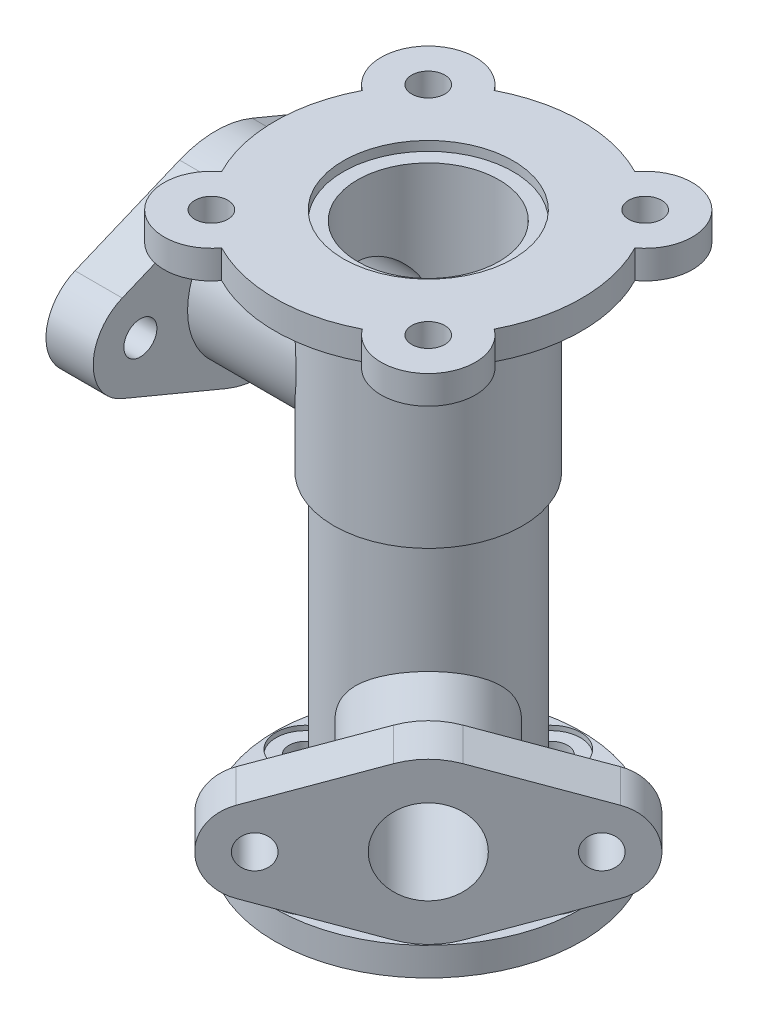
SolidWorks part; units mm, degrees
ref_plane "Front Plane" through (0, 0, 0) normal (0, 0, 1) x (1, 0, 0)
ref_plane "Top Plane" through (0, 0, 0) normal (0, 1, 0) x (1, 0, 0)
ref_plane "Right Plane" through (0, 0, 0) normal (1, 0, 0) x (0, 0, -1)
other "Configuration Table"
sketch "Sketch1" plane through (0, 0, 0) normal (0, 1, 0) x (1, 0, 0)
  circle A0 centre (0, 0) radius 32.5
  dimension "D1" = 65
extrude "Boss-Extrude1" add sketch "Sketch1" along normal blind 6
sketch "Sketch2" plane through (0, 6, 0) normal (0, 1, 0) x (1, 0, 0)
  circle A0 centre (0, 0) radius 18
  dimension "D1" = 36
extrude "Boss-Extrude2" add sketch "Sketch2" along normal blind 64
sketch "Sketch3" plane through (0, 70, 0) normal (0, 1, 0) x (1, 0, 0)
  circle A0 centre (0, 0) radius 20
  dimension "D1" = 40
extrude "Boss-Extrude3" add sketch "Sketch3" along normal blind 48
sketch "Sketch4" plane through (0, 118, 0) normal (0, 1, 0) x (1, 0, 0)
  line L0 (0, 44.6878) -> (0, 0) construction
  line L1 (0, 0) -> (32.5301, 32.5301) construction
  circle A0 centre (0, 0) radius 32.5
  circle A1 centre (22.981, 22.981) radius 10
  circle A5 centre (22.981, -22.981) radius 10
  circle A6 centre (-22.981, -22.981) radius 10
  circle A7 centre (-22.981, 22.981) radius 10
  point P16 (9.7122, 2.1531)
  point P17 (0, 0)
  circle M6 centre (0, 0) radius 20
  dimension "D1" = 65
  dimension "D2" = 20
  dimension "D3" = 45
  dimension "D4" = 4
extrude "Boss-Extrude4" add sketch "Sketch4" against normal blind 6 contours A0 A1 | A0 A1 | A7 A0 A6 A5 A1 M6 | M6 | A0 A5 | A0 A5 | A0 A6 | A0 A6
sketch "Sketch5" plane through (0, 0, 0) normal (1, 0, 0) x (0, 0, -1)
  line L0 (0, 90) -> (0, 0) construction
  circle A0 centre (0, 90) radius 16
  dimension "D2" = 32
  dimension "D1" = 90
extrude "Boss-Extrude5" add sketch "Sketch5" against normal blind 45
sketch "Sketch6" plane through (-45, 0, 0) normal (-1, 0, 0) x (0, 0, 1)
  line L0 (0, 139.4869) -> (0, 110) construction
  line L1 (0, 90) -> (47.008, 90) construction
  line L2 (7.6923, 71.5385) -> (29.8462, 80.7692)
  line L3 (7.6923, 108.4615) -> (29.8462, 99.2308)
  line L4 (-7.6923, 108.4615) -> (-29.8462, 99.2308)
  line L5 (-7.6923, 71.5385) -> (-29.8462, 80.7692)
  arc A0 (-7.6923, 71.5385) -> (7.6923, 71.5385) centre (0, 90) ccw
  arc A1 (29.8462, 80.7692) -> (29.8462, 99.2308) centre (26, 90) ccw
  arc A2 (-29.8462, 80.7692) -> (-29.8462, 99.2308) centre (-26, 90) cw
  arc A3 (7.6923, 108.4615) -> (-7.6923, 108.4615) centre (0, 90) ccw
  dimension "D1" = 40
  dimension "D2" = 20
  dimension "D3" = 52
extrude "Boss-Extrude6" add sketch "Sketch6" against normal blind 10
ref_plane "Plane1" through (0, 0, 0) normal (-0.7071, 0, 0.7071) x (0, -1, 0)
ref_plane "Plane2" through (0, 0, 0) normal (-0.7071, 0, -0.7071) x (0, -1, 0)
sketch "Sketch8" plane through (0, 0, 0) normal (-0.7071, 0, -0.7071) x (0, -1, 0)
  line L0 (-70, 0) -> (-6, 0) construction
  line L1 (-32, 0) -> (0, 0) construction
  circle A0 centre (-32, 0) radius 14
  dimension "D1" = 28
  dimension "D2" = 32
extrude "Boss-Extrude7" add sketch "Sketch8" against normal blind 45
sketch "Sketch9" plane through (31.8198, 0, 31.8198) normal (0.7071, 0, 0.7071) x (0.7071, 0, -0.7071)
  line L0 (0, 56.8043) -> (0, 32) construction
  line L1 (0, 32) -> (45.5222, 32) construction
  line L2 (5.2308, 15.8247) -> (28.7692, 23.4366)
  line L3 (5.2308, 48.1753) -> (28.7692, 40.5634)
  line L4 (-5.2308, 48.1753) -> (-28.7692, 40.5634)
  line L5 (-5.2308, 15.8247) -> (-28.7692, 23.4366)
  arc A0 (-5.2308, 15.8247) -> (5.2308, 15.8247) centre (0, 32) ccw
  arc A1 (28.7692, 23.4366) -> (28.7692, 40.5634) centre (26, 32) ccw
  arc A2 (-28.7692, 23.4366) -> (-28.7692, 40.5634) centre (-26, 32) cw
  arc A3 (5.2308, 48.1753) -> (-5.2308, 48.1753) centre (0, 32) ccw
  dimension "D1" = 18
  dimension "D2" = 34
  dimension "D3" = 52
extrude "Boss-Extrude8" add sketch "Sketch9" against normal blind 10
sketch "Sketch10" plane through (0, 0, 0) normal (0, -1, 0) x (1, 0, 0)
  circle A0 centre (0, 0) radius 13
  dimension "D1" = 26
extrude "Cut-Extrude1" cut sketch "Sketch10" against normal blind 70
sketch "Sketch11" plane through (31.8198, 0, 31.8198) normal (0.7071, 0, 0.7071) x (0.7071, 0, -0.7071)
  circle A0 centre (0, 32) radius 9
  dimension "D1" = 18
extrude "Cut-Extrude2" cut sketch "Sketch11" against normal blind 45
sketch "Sketch12" plane through (-45, 0, 0) normal (-1, 0, 0) x (0, 0, 1)
  circle A0 centre (0, 90) radius 11
  dimension "D1" = 22
extrude "Cut-Extrude3" cut sketch "Sketch12" against normal blind 45
sketch "Sketch13" plane through (0, 118, 0) normal (0, 1, 0) x (1, 0, 0)
  circle A0 centre (0, 0) radius 18
  dimension "D1" = 36
extrude "Cut-Extrude4" cut sketch "Sketch13" against normal blind 2
sketch "Sketch14" plane through (0, 116, 0) normal (0, 1, 0) x (1, 0, 0)
  circle A0 centre (0, 0) radius 15
  dimension "D1" = 30
extrude "Cut-Extrude5" cut sketch "Sketch14" against normal blind 36
sketch "Sketch15" plane through (0, 80, 0) normal (0, 1, 0) x (1, 0, 0)
  line L0 (0, -4.5826) -> (0, 4.5826) construction
  circle A0 centre (0, 0) radius 14
  dimension "D1" = 28
extrude "Cut-Extrude6" cut sketch "Sketch15" against normal blind 3
sketch "Sketch16" plane through (0, 118, 0) normal (0, 1, 0) x (1, 0, 0)
  circle A0 centre (22.981, 22.981) radius 3.5
  circle A1 centre (22.981, -22.981) radius 3.5
  circle A2 centre (-22.981, -22.981) radius 3.5
  circle A3 centre (-22.981, 22.981) radius 3.5
  point P12 (0, 0)
  dimension "D1" = 7
  dimension "D2" = 4
extrude "Cut-Extrude7" cut sketch "Sketch16" against normal blind 20
sketch "Sketch17" plane through (0, 112, 0) normal (0, -1, 0) x (1, 0, 0)
  circle A0 centre (22.981, 22.981) radius 6.5
  circle A1 centre (22.981, -22.981) radius 6.5
  circle A2 centre (-22.981, -22.981) radius 6.5
  circle A3 centre (-22.981, 22.981) radius 6.5
  point P12 (0, 0)
  dimension "D1" = 13
  dimension "D2" = 4
extrude "Cut-Extrude8" cut sketch "Sketch17" against normal blind 1
sketch "Sketch18" plane through (31.8198, 0, 31.8198) normal (0.7071, 0, 0.7071) x (0.7071, 0, -0.7071)
  circle A0 centre (-26, 32) radius 3.5
  circle A1 centre (26, 32) radius 3.5
  dimension "D1" = 7
extrude "Cut-Extrude9" cut sketch "Sketch18" against normal blind 10
sketch "Sketch19" plane through (-45, 0, 0) normal (-1, 0, 0) x (0, 0, 1)
  circle A0 centre (26, 90) radius 3.5
  circle A1 centre (-26, 90) radius 3.5
  dimension "D1" = 7
extrude "Cut-Extrude10" cut sketch "Sketch19" against normal blind 10
sketch "Sketch20" plane through (0, 0, 0) normal (0, -1, 0) x (1, 0, 0)
  circle A0 centre (0, 0) radius 26 construction
  circle A1 centre (0, -26) radius 3.5
  circle A2 centre (-26, 0) radius 3.5
  circle A3 centre (0, 26) radius 3.5
  circle A4 centre (26, 0) radius 3.5
  point P14 (0, 0)
  dimension "D1" = 52
  dimension "D2" = 7
  dimension "D3" = 4
extrude "Cut-Extrude11" cut sketch "Sketch20" against normal blind 20
sketch "Sketch21" plane through (0, 6, 0) normal (0, 1, 0) x (1, 0, 0)
  circle A0 centre (-26, 0) radius 6.25
  circle A1 centre (0, 26) radius 6.25
  circle A2 centre (26, 0) radius 6.25
  circle A3 centre (0, -26) radius 6.25
  point P11 (0, 0)
  dimension "D1" = 12.5
  dimension "D2" = 4
extrude "Cut-Extrude12" cut sketch "Sketch21" against normal blind 1
sketch "Sketch22" plane through (0, 77, 0) normal (0, 1, 0) x (1, 0, 0)
  circle A0 centre (0, 0) radius 10
  dimension "D1" = 20
extrude "Cut-Extrude13" cut sketch "Sketch22" against normal blind 50
